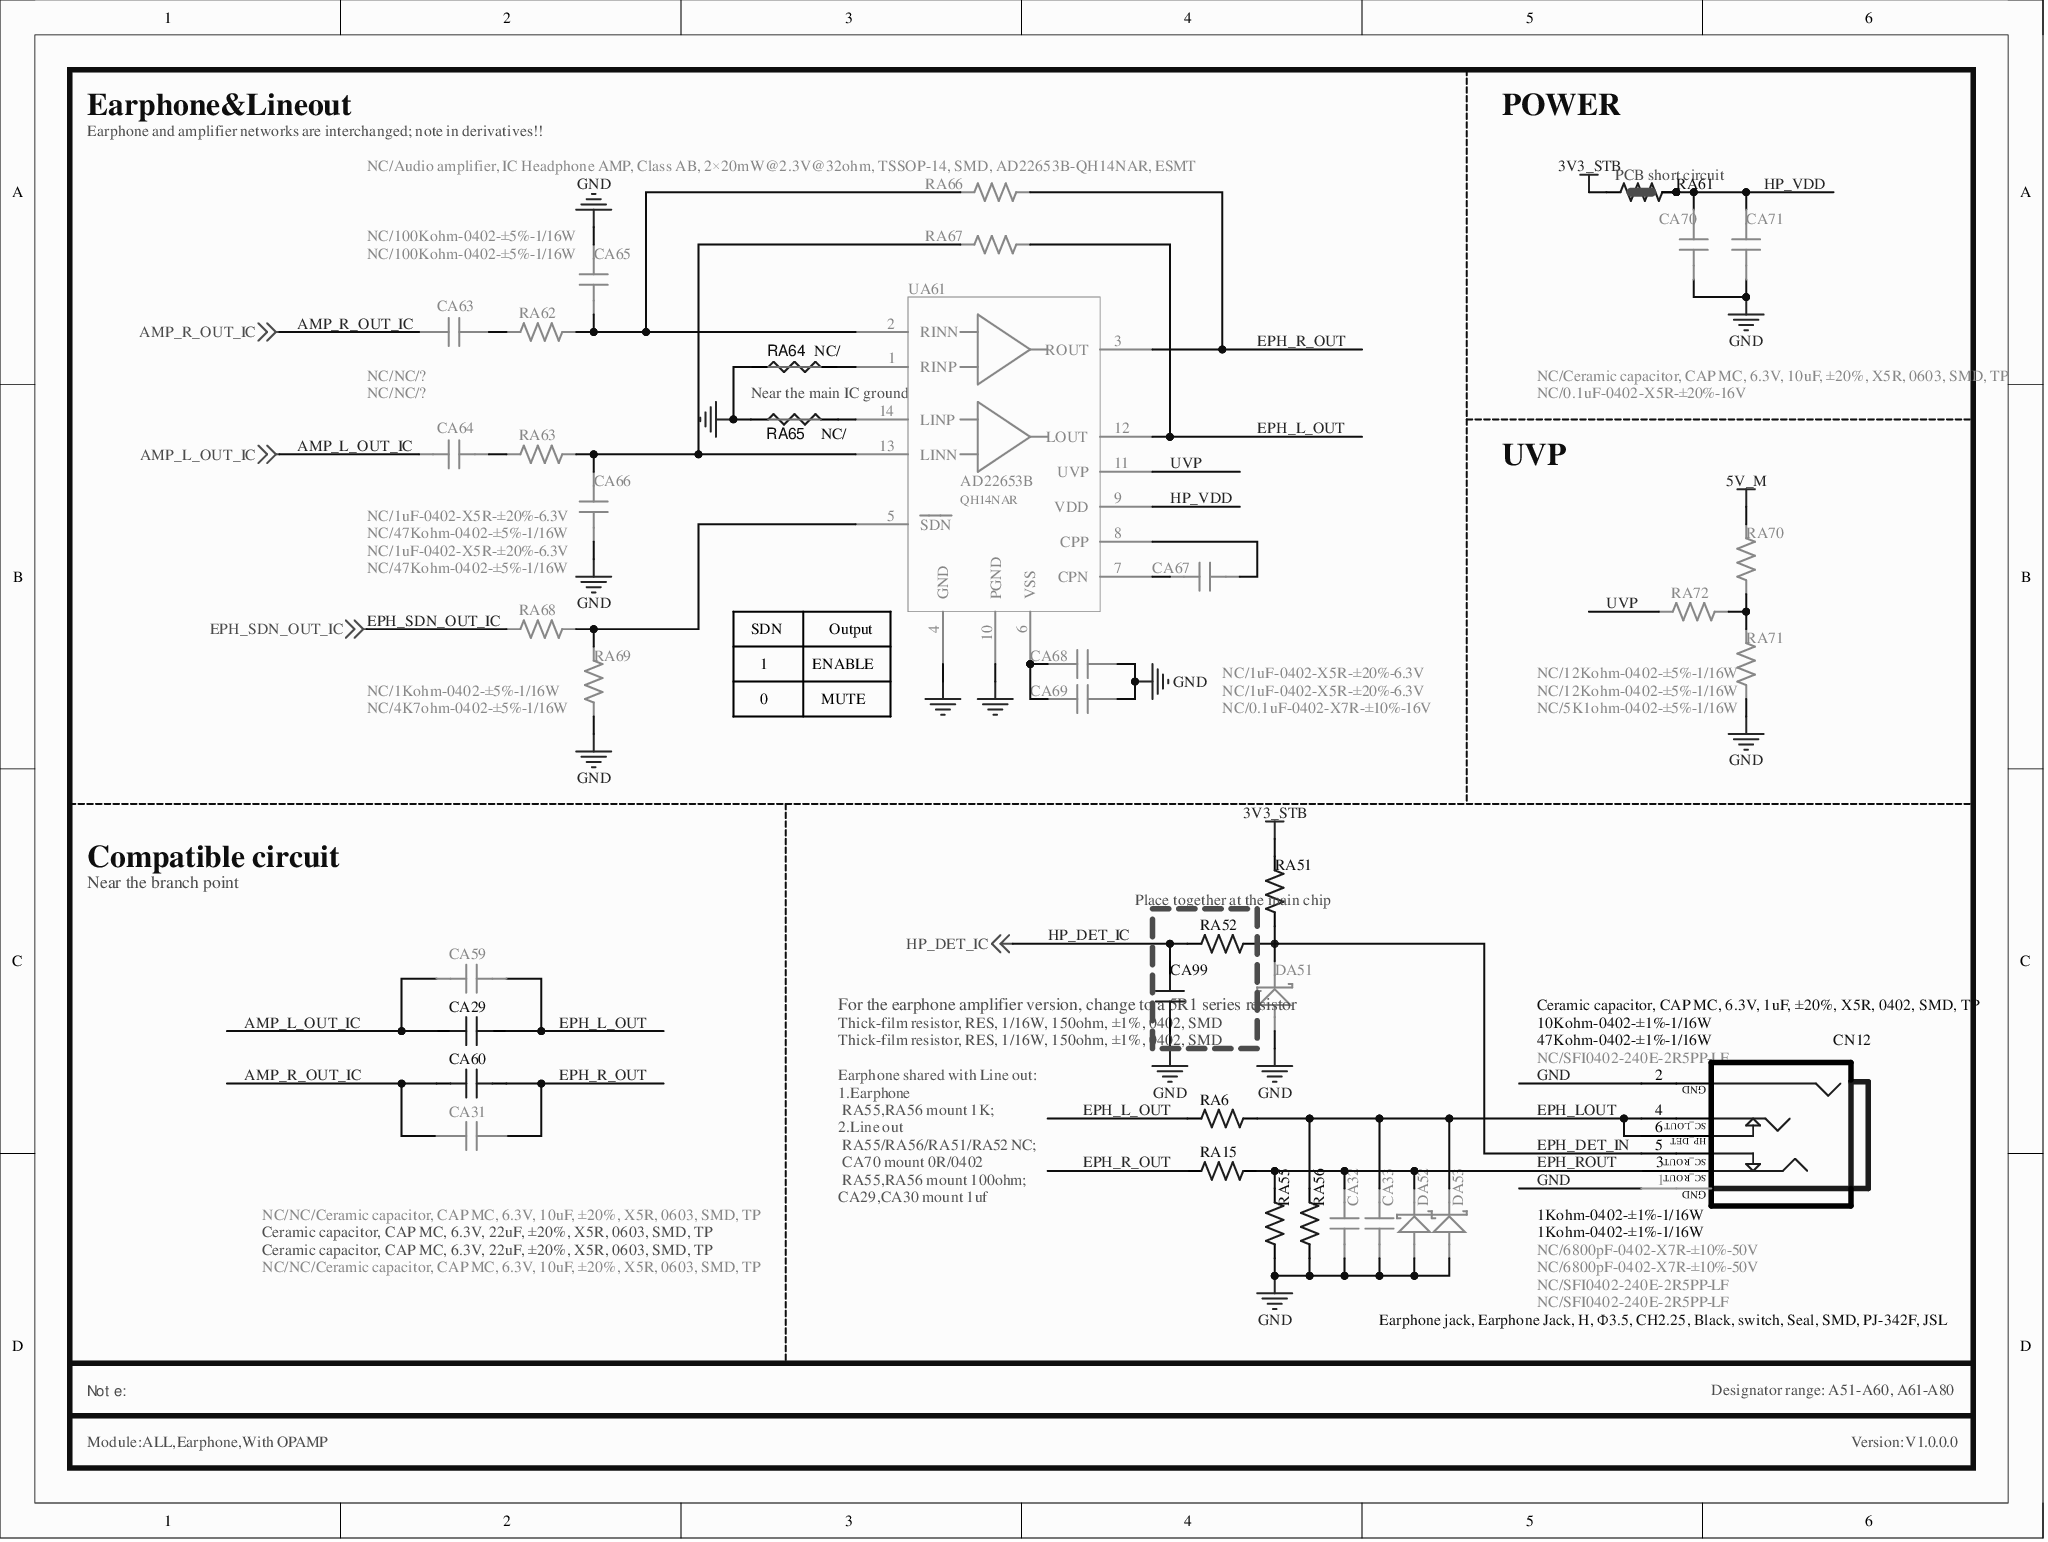
[diagram p0: MISC105950-44.SchDoc]
# Altium project MISC105950-48.PrjPCB (part 7 of 8)
## Sheet MISC105950-44.SchDoc
size 297 x 223 mm

### Parts
CA29  Ceramic capacitor, CAP MC, 6.3V, 22uF, ±20%, X5R, 0603, SMD, TP  [C0603]
CA31  NC/NC/Ceramic capacitor, CAP MC, 6.3V, 10uF, ±20%, X5R, 0603, SMD, TP  [C0603]
CA32  NC/6800pF-0402-X7R-±10%-50V  [C0402]
CA33  NC/6800pF-0402-X7R-±10%-50V  [C0402]
CA59  NC/NC/Ceramic capacitor, CAP MC, 6.3V, 10uF, ±20%, X5R, 0603, SMD, TP  [C0603]
CA60  Ceramic capacitor, CAP MC, 6.3V, 22uF, ±20%, X5R, 0603, SMD, TP  [C0603]
CA63  NC/1uF-0402-X5R-±20%-6.3V  [C0402]
CA64  NC/1uF-0402-X5R-±20%-6.3V  [C0402]
CA65  NC/NC/?  [C0402]
CA66  NC/NC/?  [C0402]
CA67  NC/1uF-0402-X5R-±20%-6.3V  [C0402]
CA68  NC/1uF-0402-X5R-±20%-6.3V  [C0402]
CA69  NC/0.1uF-0402-X7R-±10%-16V  [C0402]
CA70  NC/Ceramic capacitor, CAP MC, 6.3V, 10uF, ±20%, X5R, 0603, SMD, TP  [C0603]
CA71  NC/0.1uF-0402-X5R-±20%-16V  [C0402]
CA99  Ceramic capacitor, CAP MC, 6.3V, 1uF, ±20%, X5R, 0402, SMD, TP  [C0402]
CN12  Earphone jack, Earphone Jack, H, Φ3.5, CH2.25, Black, switch, Seal, SMD, PJ-342F, JSL  [PHONE-HS-29]
DA51  NC/SFI0402-240E-2R5PP-LF  [DIODE-S0402]
DA52  NC/SFI0402-240E-2R5PP-LF  [DIODE-S0402]
DA53  NC/SFI0402-240E-2R5PP-LF  [DIODE-S0402]
RA6  Thick-film resistor, RES, 1/16W, 150ohm, ±1%, 0402, SMD  [R0402]
RA15  Thick-film resistor, RES, 1/16W, 150ohm, ±1%, 0402, SMD  [R0402]
RA51  47Kohm-0402-±1%-1/16W  [R0402]
RA52  10Kohm-0402-±1%-1/16W  [R0402]
RA55  1Kohm-0402-±1%-1/16W  [R0402]
RA56  1Kohm-0402-±1%-1/16W  [R0402]
RA61  NC/NC/0ohm-0402-PCB  [R0402SC]  (value not drawn)
RA62  NC/47Kohm-0402-±5%-1/16W  [R0402]
RA63  NC/47Kohm-0402-±5%-1/16W  [R0402]
RA64  NC/  [GND]
RA65  NC/  [GND]
RA66  NC/100Kohm-0402-±5%-1/16W  [R0402]
RA67  NC/100Kohm-0402-±5%-1/16W  [R0402]
RA68  NC/1Kohm-0402-±5%-1/16W  [R0402]
RA69  NC/4K7ohm-0402-±5%-1/16W  [R0402]
RA70  NC/12Kohm-0402-±5%-1/16W  [R0402]
RA71  NC/5K1ohm-0402-±5%-1/16W  [R0402]
RA72  NC/12Kohm-0402-±5%-1/16W  [R0402]
UA61  NC/Audio amplifier, IC Headphone AMP, Class AB, 2×20mW@2.3V@32ohm, TSSOP-14, SMD, AD22653B-QH14NAR, ESMT  [SSOP14/0.65-1]

### Nets
3V3_STB: RA51.2 RA61.1
5V_M: RA70.2
GND: CA32.2 CA33.2 CA65.2 CA66.1 CA68.2 CA69.2 CA70.2 CA71.2 CA99.1 CN12.1 CN12.2 DA51.A DA52.A DA53.A RA55.1 RA56.1 RA64.JP_2K RA65.JP_2K RA69.1 RA71.1 UA61.4(GND) UA61.10(PGND)
AMP_L_OUT_IC: CA29.1 CA59.1 CA64.1 ; off-sheet AMP_L_OUT_IC
AMP_R_OUT_IC: CA31.1 CA60.1 CA63.1 ; off-sheet AMP_R_OUT_IC
EPH_DET_IN: CN12.5 DA51.K RA51.1 RA52.1
EPH_L_OUT: CA29.2 CA59.2 RA6.1 RA67.2 UA61.12(LOUT)
EPH_LOUT: CA33.1 CN12.4 CN12.6 DA53.K RA6.2 RA56.2
EPH_R_OUT: CA31.2 CA60.2 RA15.1 RA66.2 UA61.3(ROUT)
EPH_ROUT: CA32.1 CN12.3 DA52.K RA15.2 RA55.2
EPH_SDN_OUT_IC: RA68.1 ; off-sheet EPH_SDN_OUT_IC
HP_DET_IC: CA99.2 RA52.2 ; off-sheet HP_DET_IC
HP_VDD: CA70.1 CA71.1 RA61.2 RA61.3 UA61.9(VDD)
UVP: RA72.2 UA61.11(UVP)
NetCA63_2: CA63.2 RA62.1
NetCA64_2: CA64.2 RA63.1
NetCA65_1: CA65.1 RA62.2 RA66.1 UA61.2(RINN)
NetCA66_2: CA66.2 RA63.2 RA67.1 UA61.13(LINN)
NetCA67_1: CA67.1 UA61.8(CPP)
NetCA67_2: CA67.2 UA61.7(CPN)
NetCA68_1: CA68.1 CA69.1 UA61.6(VSS)
NetRA64_JP_1K: RA64.JP_1K UA61.1(RINP)
NetRA65_JP_1K: RA65.JP_1K UA61.14(LINP)
NetRA68_2: RA68.2 RA69.2 UA61.5(~{SDN})
NetRA70_1: RA70.1 RA71.2 RA72.1

### Notes on the sheet
- Earphone&Lineout
- Earphone and amplifier networks are interchanged; note in derivatives!!
- POWER
- (near UA61) Near the main IC ground
- UVP
- SDN
- 1
- 0
- (near UA61) ENABLE
- MUTE
- (near UA61) Output
- Compatible circuit
- Near the branch point
- (near RA51) Place together at the main chip
- For the earphone amplifier version, change to a 5R1 series resistor
- Earphone shared with Line out:
  1.Earphone
  RA55,RA56 mount 1K;
  2.Line out
  RA55/RA56/RA51/RA52 NC;
  CA70 mount 0R/0402
  RA55,RA56 mount 100ohm;
  CA29,CA30 mount 1uf
- Note:
- Designator range: A51-A60, A61-A80
- Module:ALL,Earphone,With OPAMP
- Version:V1.0.0.0

### Library data of the parts
CA29 CA31 CA59 CA60 = 22uF-0603-X5R-±20%-6.3V-D
CA32 CA33 CA63 CA64 CA67 = 004.003.0000382-D: Ceramic capacitor, CAP MC, 6.3V, 1uF, ±20%, X5R, 0402, SMD, TP-D
CA65 CA66 = 004.003.0000532-D: Ceramic capacitor, CAP MC, 50V, 220pF, ±5%, NPO, 0402, SMD, TP-D
CA68 = 004.003.0000100-D: Ceramic capacitor, CAP MC, 6.3V, 2.2uF, ±20%, X5R, 0402, SMD, TP-D
CA69 = 004.003.0000403-D: as CA8 on sheet MISC105950-41
CA70 = 004.003.0000383-D: Ceramic capacitor, CAP MC, 6.3V, 10uF, ±20%, X5R, 0603, SMD, TP-D
CA71 = 0.1uF-0402-X5R-±20%-16V-D
CA99 = 1uF-0402-X5R-±20%-6.3V-D
CN12 = XXX.XXX.0004228-D: Earphone jack, Earphone Jack, H, Φ3.5, CH2.25, Black, switch, Seal, SMD, PJ-342F, JSL-D
DA51-DA53 = 004.005.0000315-D: as DH1-DH4 on sheet MISC105950-40
RA6 RA15 = 004.002.0000715-D: Thick-film resistor, RES, 1/16W, 5.1ohm, ±5%, 0402, SMD-D
RA51 RA62 RA63 = 004.002.0000691-D: as RA9 on sheet MISC105950-41
RA52 = 004.002.0000577-D: Thick-film resistor, RES, 1/16W, 10Kohm, ±5%, 0402, SMD-D
RA55 RA56 RA68 = 004.002.0000572-D: as RA3 on sheet MISC105950-41
RA61 = 0ohm-0402-PCB-D
RA64 RA65 = GND: as RA4 on sheet MISC105950-41
RA66 RA67 = 004.002.0000579-D: as RA8 on sheet MISC105950-41
RA69 RA71 = 004.002.0000689-D: as RA1 on sheet MISC105950-41
RA70 RA72 = 004.002.0000589-D: Thick-film resistor, RES, 1/16W, 12Kohm, ±5%, 0402, SMD-D
UA61 = 004.012.0000155-D: Audio amplifier, IC Headphone AMP, Class AB, 2×20mW@2.3V@32ohm, TSSOP-14, SMD, AD22653B-QH14NAR, ESMT-D